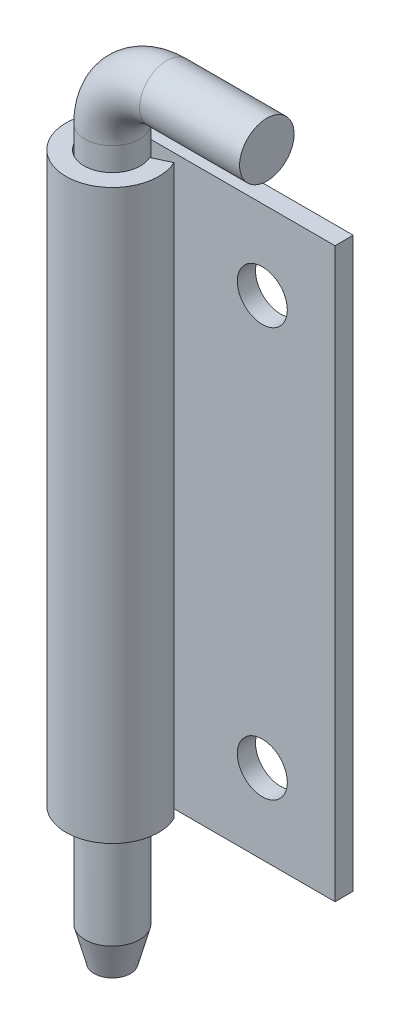
SolidWorks part; units mm, degrees
ref_plane "前视" through (0, 0, 0) normal (0, 0, 1) x (1, 0, 0)
ref_plane "上视" through (0, 0, 0) normal (0, 1, 0) x (1, 0, 0)
ref_plane "右视" through (0, 0, 0) normal (1, 0, 0) x (0, 0, -1)
sketch "草图1" plane through (0, 0, 0) normal (0, 0, 1) x (1, 0, 0)
  line L0 (0, 0) -> (0, 80)
  line L1 (6, 86) -> (17, 86)
  arc A0 (0, 80) -> (6, 86) centre (6, 80) cw
  point P6 (0, 86)
  dimension "D3" = 6
  dimension "D1" = 17
  dimension "D2" = 86
sketch "草图2" plane through (0, 0, 0) normal (0, 1, 0) x (1, 0, 0)
  circle A0 centre (0, 0) radius 3
  dimension "D1" = 6
sweep "扫描1" add profiles "草图2" path "草图1"
ref_plane "基准面1" through (0, 15, 0) normal (0, -1, 0) x (-1, 0, 0)
sketch "草图3" plane through (0, 15, 0) normal (0, -1, 0) x (-1, 0, 0)
  line L0 (0, 3.1) -> (-21.4, 3.1)
  line L1 (0, 5.1) -> (-21.4, 5.1)
  line L2 (0, 0) -> (0, 2.8615) construction
  line L3 (0, 0) -> (-4.3836, 2.0441) construction
  line L4 (-2.8096, 1.3101) -> (-4.6222, 2.1554)
  line L5 (-21.4, 3.1) -> (-21.4, 5.1)
  arc A0 (-2.8096, 1.3101) -> (0, 3.1) centre (0, 0) ccw
  arc A1 (-4.6222, 2.1554) -> (0, 5.1) centre (0, 0) ccw
  arc A3 (-1.7443, 4.7924) -> (0, 5.1) centre (0, 0) ccw construction
  arc A4 (-1.0603, 2.913) -> (0, 3.1) centre (0, 0) ccw construction
  dimension "D1" = 6.2
  dimension "D2" = 21.4
  dimension "D3" = 2
  dimension "D4" = 65
extrude "凸台-拉伸1" add sketch "草图3" against normal blind 62.5
sketch "草图5" plane through (0, 0, -3.1) normal (0, 0, 1) x (1, 0, 0)
  line L0 (21.4, 77.5) -> (21.4, 15) construction
  line L1 (21.4, 46.25) -> (-13.6129, 46.25) construction
  circle A0 centre (13.4, 23.75) radius 2.75
  circle A1 centre (13.4, 68.75) radius 2.75
  dimension "D1" = 8
  dimension "D2" = 45
  dimension "D3" = 5.5
extrude "切除-拉伸2" cut sketch "草图5" against normal through all
chamfer "倒角1" distance 1 angle 75 1 edges at (0, 0, 3)
